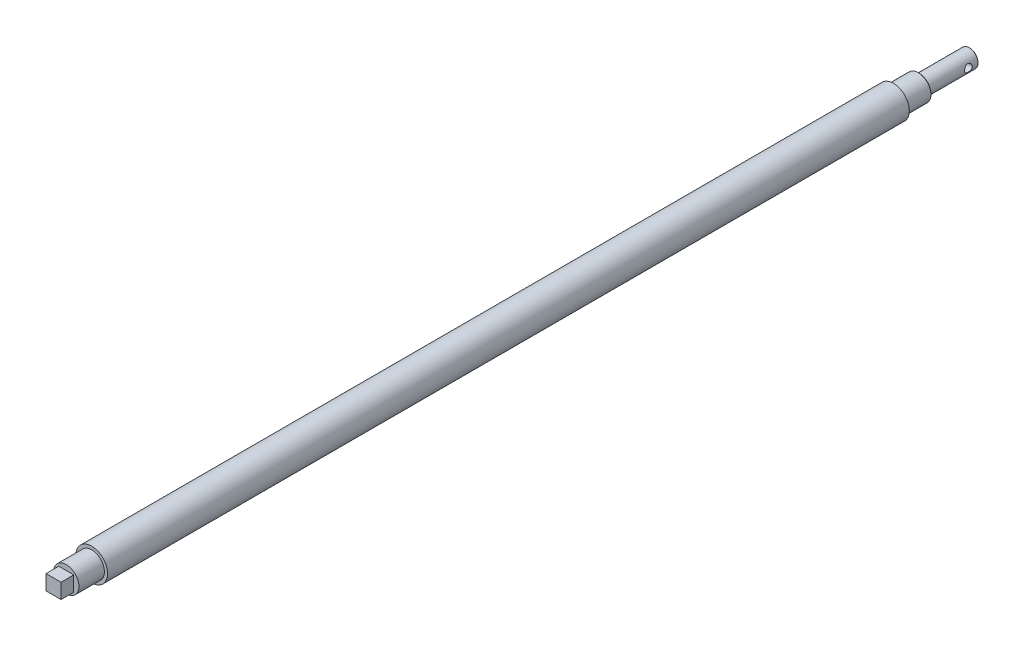
SolidWorks part; units mm, degrees
material "45#"
ref_plane "前基準面" through (0, 0, 0) normal (0, 0, 1) x (1, 0, 0)
ref_plane "上基準面" through (0, 0, 0) normal (0, 1, 0) x (1, 0, 0)
ref_plane "右基準面" through (0, 0, 0) normal (1, 0, 0) x (0, 0, -1)
sketch "草图1" plane through (0, 0, 0) normal (0, 0, 1) x (1, 0, 0)
  circle A0 centre (0, 0) radius 12.5
  dimension "D1" = 25
extrude "凸台-拉伸1" add sketch "草图1" along normal mid plane 630
sketch "草图2" plane through (0, 0, 315) normal (0, 0, 1) x (1, 0, 0)
  circle A0 centre (0, 0) radius 10
  dimension "D1" = 20
extrude "凸台-拉伸2" add sketch "草图2" along normal blind 30
sketch "草图3" plane through (0, 0, -315) normal (0, 0, -1) x (-1, 0, 0)
  circle A0 centre (0, 0) radius 10
  circle A1 centre (0, 0) radius 10 construction
extrude "凸台-拉伸3" add sketch "草图3" along normal blind 20
chamfer "倒角1" distance 0.5 angle 45 2 edges at (-10, 0, -335) (10, 0, 345)
sketch "草图4" plane through (0, 0, -335) normal (0, 0, -1) x (-1, 0, 0)
  circle A0 centre (0, 0) radius 7
  dimension "D1" = 14
extrude "凸台-拉伸4" add sketch "草图4" along normal blind 40
chamfer "倒角2" distance 0.5 angle 45 1 edges at (-7, 0, -375)
sketch "草图5" plane through (0, 0, 0) normal (1, 0, 0) x (0, 0, -1)
  line L0 (375, -6.5) -> (375, 6.5) construction
  circle A0 centre (367, 0) radius 3
  dimension "D1" = 6
  dimension "D2" = 8
extrude "切除-拉伸1" cut sketch "草图5" against normal through all both and the other way through all
sketch "草图6" plane through (0, 0, 345) normal (0, 0, 1) x (1, 0, 0)
  line L1 (-5.9, -5.9) -> (5.9, -5.9)
  line L2 (-5.9, -5.9) -> (-5.9, 5.9)
  line L3 (-5.9, 5.9) -> (5.9, 5.9)
  line L4 (5.9, -5.9) -> (5.9, 5.9)
  line L5 (-5.9, -5.9) -> (5.9, 5.9) construction
  line L6 (-5.9, 5.9) -> (5.9, -5.9) construction
  circle A0 centre (0, 0) radius 16.9378
  point P0 (0, 0)
  dimension "D1" = 11.8
extrude "切除-拉伸2" cut sketch "草图6" against normal blind 10
